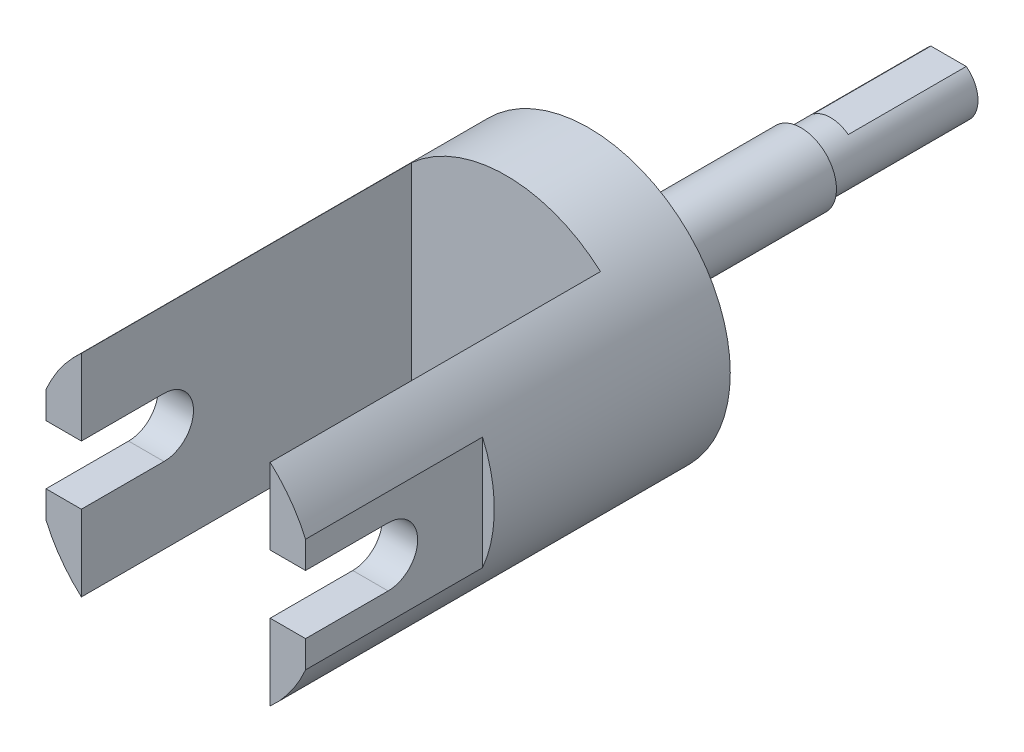
SolidWorks part; units mm, degrees
ref_plane "Front Plane" through (0, 0, 0) normal (0, 0, 1) x (1, 0, 0)
ref_plane "Top Plane" through (0, 0, 0) normal (0, 1, 0) x (1, 0, 0)
ref_plane "Right Plane" through (0, 0, 0) normal (1, 0, 0) x (0, 0, -1)
sketch "Sketch1" plane through (0, 0, 0) normal (0, 0, 1) x (1, 0, 0)
  circle A0 centre (0, 0) radius 12
  dimension "D1" = 24
extrude "Boss-Extrude1" add sketch "Sketch1" along normal blind 35
sketch "Sketch2" plane through (0, 0, 0) normal (0, 0, -1) x (-1, 0, 0)
  circle A0 centre (0, 0) radius 3.5
  dimension "D1" = 7
extrude "Boss-Extrude2" add sketch "Sketch2" along normal blind 5
sketch "Sketch3" plane through (0, 0, 35) normal (0, 0, 1) x (1, 0, 0)
  line L1 (-8, 12.5) -> (8, 12.5)
  line L2 (-8, 12.5) -> (-8, -12.5)
  line L3 (-8, -12.5) -> (8, -12.5)
  line L4 (8, 12.5) -> (8, -12.5)
  line L5 (-8, 12.5) -> (8, -12.5) construction
  line L6 (-8, -12.5) -> (8, 12.5) construction
  point P1 (0, 0)
  dimension "D1" = 16
  dimension "D2" = 25
extrude "Cut-Extrude1" cut sketch "Sketch3" against normal blind 28
sketch "Sketch4" plane through (0, 0, 0) normal (1, 0, 0) x (0, 0, -1)
  line L0 (-28, -2.5) -> (-35, -2.5)
  line L2 (-35, -2.5) -> (-35, 2.5)
  line L3 (-35, 2.5) -> (-28, 2.5)
  line L4 (-35, 8.9443) -> (-35, -8.9443) construction
  arc A0 (-28, -2.5) -> (-28, 2.5) centre (-28, 0) ccw
  dimension "D2" = 5
  dimension "D1" = 7
extrude "Cut-Extrude2" cut sketch "Sketch4" against normal mid plane 30
sketch "Sketch5" plane through (0, 0, 35) normal (0, 0, 1) x (1, 0, 0)
  line L4 (11, -4.7958) -> (11, 4.7958)
  line L5 (0, 0) -> (0, -12) construction
  line L7 (8, -8.9443) -> (8, -2.5) construction
  line L8 (-11, -4.7958) -> (-11, 4.7958)
  arc A7 (11, -4.7958) -> (11, 4.7958) centre (0, 0) ccw
  arc A9 (-8, -8.9443) -> (8, -8.9443) centre (0, 0) ccw construction
  arc A10 (-11, -4.7958) -> (-11, 4.7958) centre (0, 0) cw
  dimension "D1" = 3
extrude "Cut-Extrude3" cut sketch "Sketch5" against normal blind 15
sketch "Sketch6" plane through (0, 0, -5) normal (0, 0, -1) x (-1, 0, 0)
  circle A0 centre (0, 0) radius 3
  dimension "D1" = 6
extrude "Boss-Extrude3" add sketch "Sketch6" along normal blind 13
sketch "Sketch7" plane through (0, 0, -18) normal (0, 0, -1) x (-1, 0, 0)
  circle A0 centre (0, 0) radius 2.5
extrude "Boss-Extrude4" add sketch "Sketch7" along normal blind 12.5
ref_plane "Plane1" through (0, 3, 0) normal (0, 1, 0) x (1, 0, 0)
sketch "Sketch8" plane through (0, 0, -30.5) normal (0, 0, -1) x (-1, 0, 0)
  line L1 (-4.5158, 2) -> (4.5158, 2)
  line L2 (-4.5158, 2) -> (-4.5158, 4.524)
  line L3 (-4.5158, 4.524) -> (4.5158, 4.524)
  line L4 (4.5158, 2) -> (4.5158, 4.524)
  line L5 (-4.5158, 2) -> (4.5158, 4.524) construction
  line L6 (-4.5158, 4.524) -> (4.5158, 2) construction
  point P0 (0, 3.262)
  dimension "D1" = 2
extrude "Cut-Extrude4" cut sketch "Sketch8" against normal blind 10
